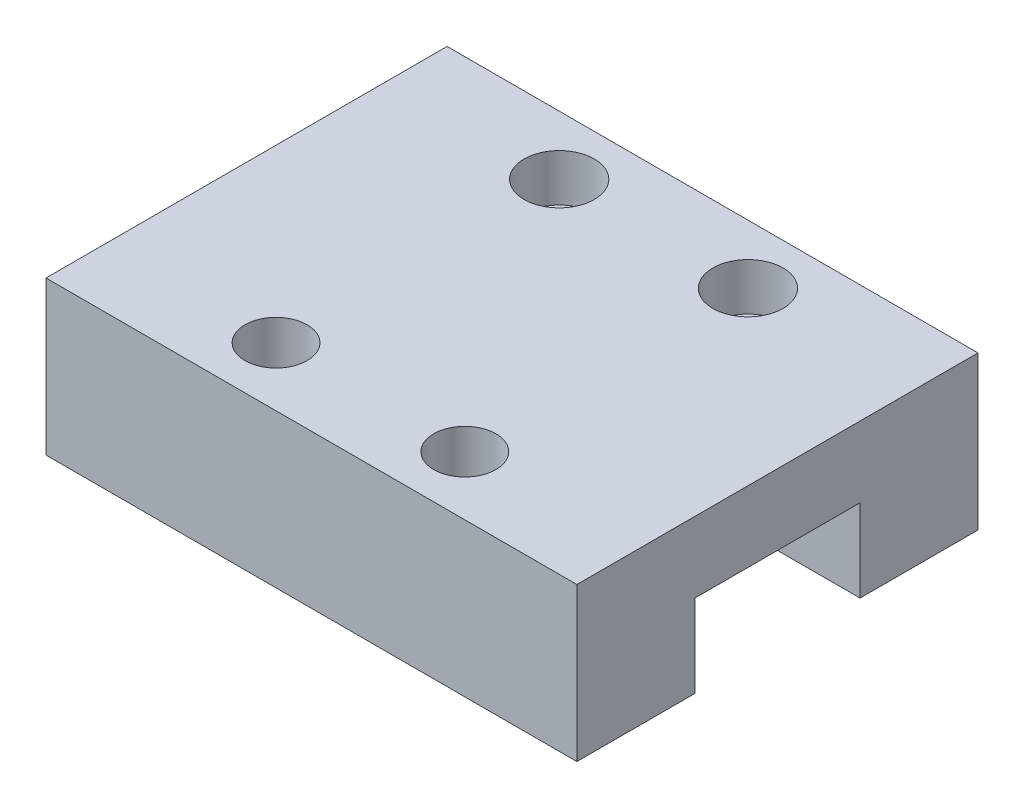
from build123d import *

# Parameters (mm, degrees)
BOSS_EXTRUDE1_DEPTH = 11.25
SKETCH2_R           = 1.317449136
SKETCH2_R_2         = 1.488469479
CUT_EXTRUDE1_DEPTH  = 2


with BuildPart() as part:
    # Sketch1 → Boss-Extrude1 (new, symmetric)
    with BuildSketch(Plane(origin=(0, 0, 0), x_dir=(0, 0, -1), z_dir=(1, 0, 0))):
        Polygon((-8.258522727, 5.046875), (8.741477273, 5.046875), (8.741477273, -1.453125), (3.741477273, -1.453125), (3.741477273, 2.046875), (-3.258522727, 2.046875), (-3.258522727, -1.453125), (-8.258522727, -1.453125), align=None)
    extrude(amount=BOSS_EXTRUDE1_DEPTH, both=True)

    # Sketch2 → Cut-Extrude1 (cut)
    with BuildSketch(Plane(origin=(0, 5.046875, 0), x_dir=(1, 0, 0), z_dir=(0, 1, 0))):
        with Locations(Location((4, -5.758522727, 0), (0, 0, 270))):
            Circle(SKETCH2_R)
        with Locations(Location((-4, 6.241477273, 0), (0, 0, 270))):
            Circle(SKETCH2_R_2)
        with Locations(Location((4, 6.241477273, 0), (0, 0, 90))):
            Circle(SKETCH2_R_2)
        with Locations(Location((-4, -5.758522727, 0), (0, 0, 90))):
            Circle(SKETCH2_R)
    extrude(amount=-CUT_EXTRUDE1_DEPTH, mode=Mode.SUBTRACT)


solid = part.part
